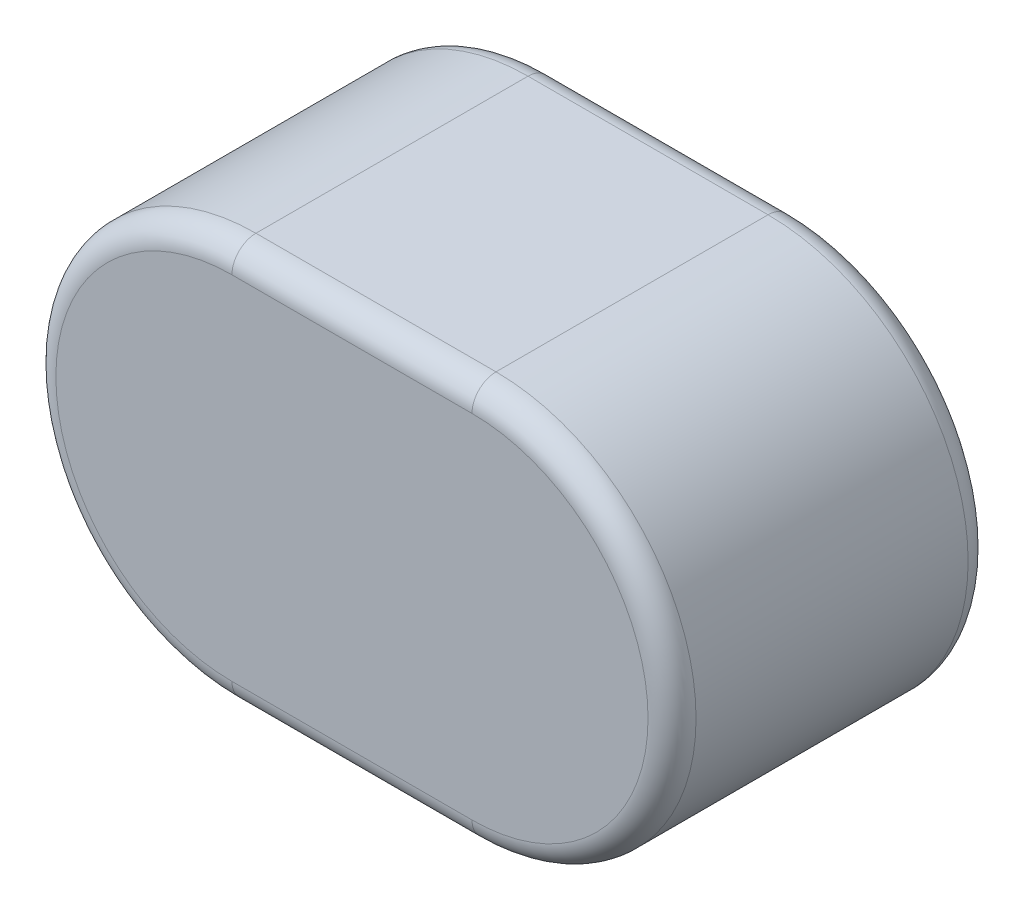
SolidWorks part; units mm, degrees
material "45"
ref_plane "基准面1" through (0, 0, 0) normal (0, 0, 1) x (1, 0, 0)
ref_plane "基准面2" through (0, 0, 0) normal (0, 1, 0) x (1, 0, 0)
ref_plane "基准面3" through (0, 0, 0) normal (1, 0, 0) x (0, 0, -1)
sketch "尺寸草图" plane through (0, 0, 0) normal (0, 0, 1) x (1, 0, 0)
  line L0 (-8, 0) -> (8, 0) construction
  point P3 (-8, 0)
  point P4 (-0.6, 0)
  point P5 (0, 0)
  point P8 (-10, 0)
  point P11 (0, 0)
sketch "草图1" plane through (0, 0, 0) normal (0, 0, 1) x (1, 0, 0)
  line L0 (-28.0599, 0) -> (30.562, 0) construction
  line L1 (-3, 5) -> (3, 5)
  line L2 (-3, -5) -> (3, -5)
  line L3 (0, 2.9108) -> (0, -2.1805) construction
  arc A0 (-3, 5) -> (-3, -5) centre (-3, 0) ccw
  arc A1 (3, 5) -> (3, -5) centre (3, 0) cw
extrude "基体-拉伸" add sketch "草图1" along normal blind 8
fillet "圆角1" radius 0.6 8 edges at (8, 0, 8) (0, 5, 8) (-8, 0, 8) (0, 5, 0) (8, 0, 0) (0, -5, 0) (-8, 0, 0) (0, -5, 8)
equation "\"D3@草图1\" = \"L@尺寸草图\""
equation "\"D1@草图1\" = \"b@尺寸草图\" / 2"
equation "\"D1@圆角1\" = \"r@尺寸草图\""
equation "\"D1@基体-拉伸\" = \"h@尺寸草图\""
